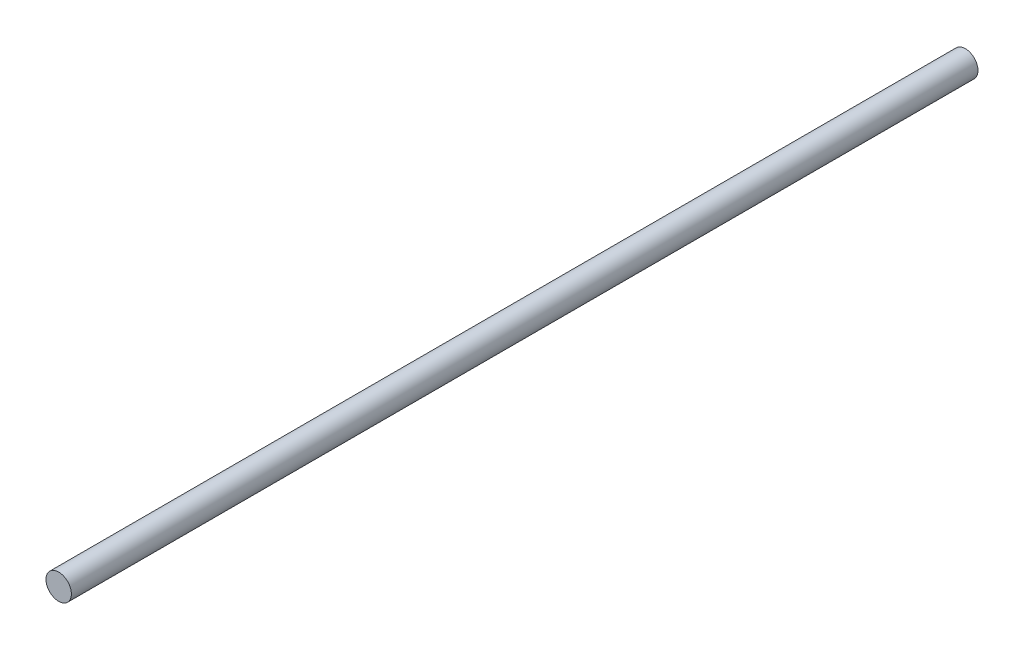
from build123d import *

# Parameters (mm, degrees)
SKETCH1_R           = 2.5
BOSS_EXTRUDE1_DEPTH = 178.5


with BuildPart() as part:
    # Sketch1 → Boss-Extrude1 (new body)
    with BuildSketch(Plane.XY):
        Circle(SKETCH1_R)
    extrude(amount=BOSS_EXTRUDE1_DEPTH)


solid = part.part
